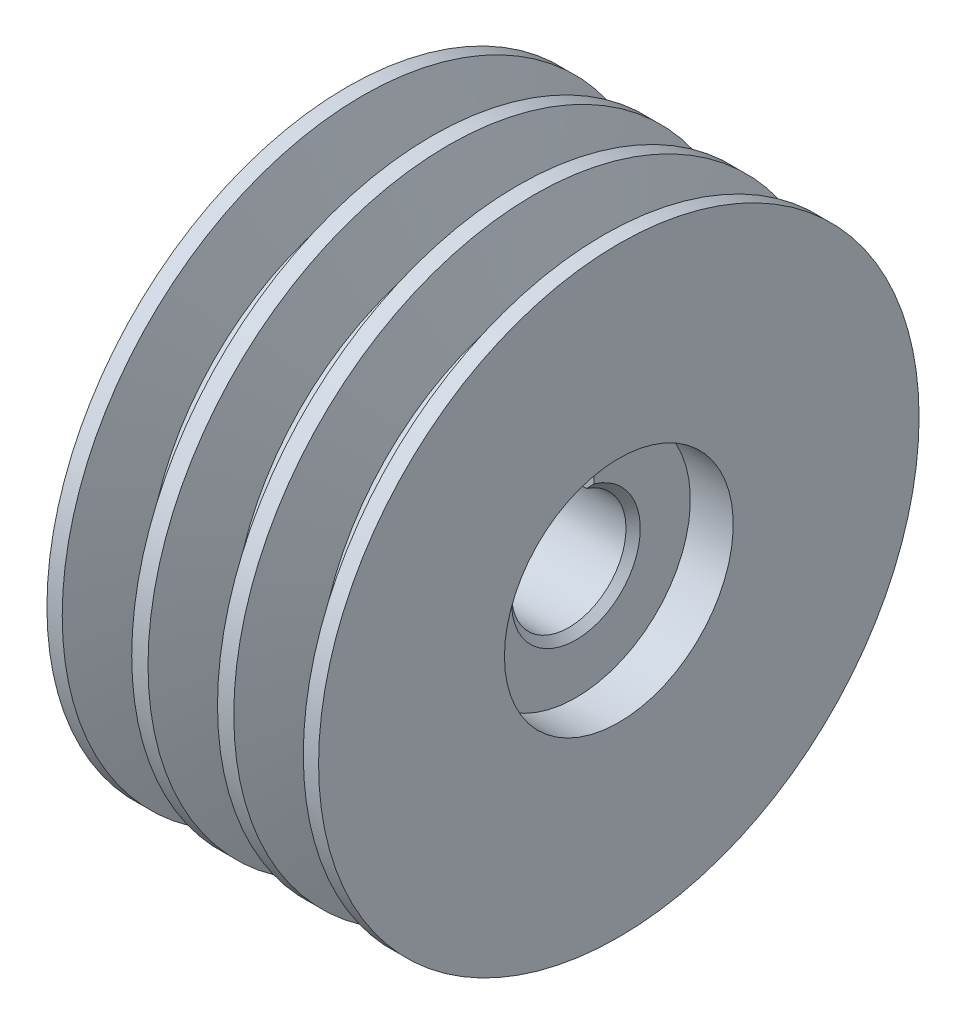
from build123d import *

# Parameters (mm, degrees)
PATTERN_LINEAR_1_COUNT = 3
PATTERN_LINEAR_1_PITCH = 12
CHAMFER_1_SIZE         = 1
SKETCH_4_W             = 5
SKETCH_4_H             = 2.700657875
CUT_EXTRUDE_1_DEPTH    = 71.512410255


with BuildPart() as part:
    # 草图1 → 旋转1 (revolve)
    with BuildSketch(Plane.XY, mode=Mode.PRIVATE) as revolve_1_sk:
        Polygon((0, 8), (0, 42), (38, 42), (38, 16), (32, 16), (32, 8), align=None)
    revolve(revolve_1_sk.sketch.rotate(Axis((0, 0, 0), (1, 0, 0)), 90), axis=Axis((0, 0, 0), (1, 0, 0)))

    # 草图2 → 切除-旋转1 (revolve, cut)
    with BuildSketch(Plane.XY, mode=Mode.PRIVATE) as cut_revolve_1_sk:
        Polygon((9.10988523, 33), (11.861461363, 42), (2.138538637, 42), (4.89011477, 33), align=None)
    cut_revolve_1 = revolve(cut_revolve_1_sk.sketch.rotate(Axis((0, 0, 0), (1, 0, 0)), 90), axis=Axis((0, 0, 0), (1, 0, 0)), mode=Mode.SUBTRACT)

    # 阵列(线性)1: 切除-旋转1 ×3
    with Locations(*[(i * PATTERN_LINEAR_1_PITCH, 0, 0) for i in range(1, PATTERN_LINEAR_1_COUNT)]):
        add(cut_revolve_1, mode=Mode.SUBTRACT)

    # 倒角1
    chamfer_1_edges = [part.edges().sort_by_distance(p)[0] for p in [
        (32, 0, -8),
        (0, 0, -8),
    ]]
    chamfer(chamfer_1_edges, length=CHAMFER_1_SIZE)

    # 草图4 → 切除-拉伸1 (cut, through all)
    with BuildSketch(Plane.ZY):
        with Locations((0, 8.949671014)):
            Rectangle(SKETCH_4_W, SKETCH_4_H)
    extrude(amount=-CUT_EXTRUDE_1_DEPTH, mode=Mode.SUBTRACT)


solid = part.part
